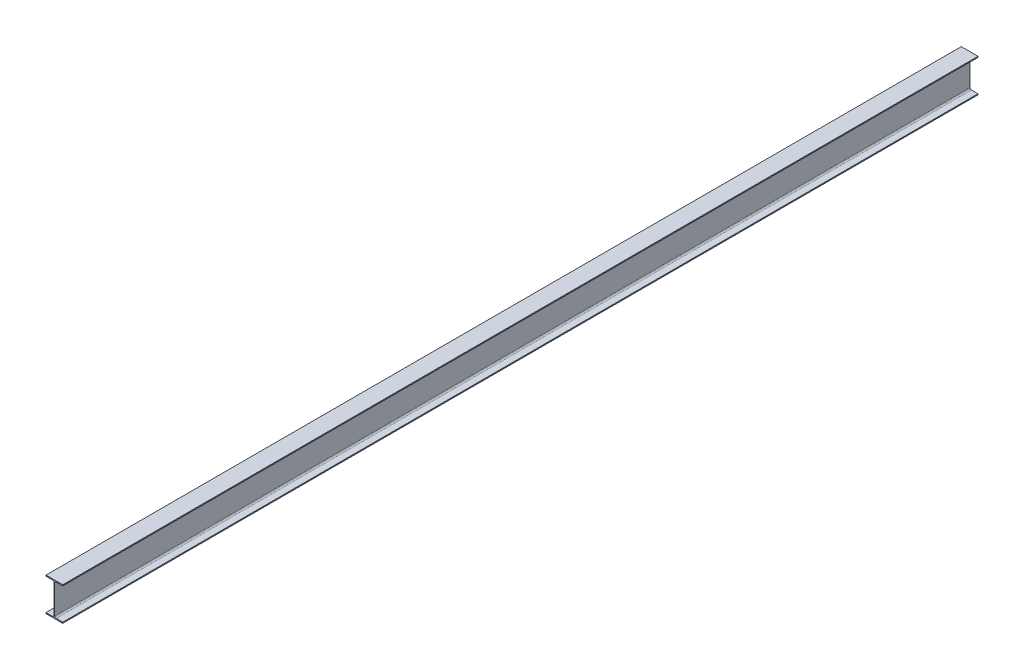
SolidWorks part; units mm, degrees
ref_plane "Front Plane" through (0, 0, 0) normal (0, 0, 1) x (1, 0, 0)
ref_plane "Top Plane" through (0, 0, 0) normal (0, 1, 0) x (1, 0, 0)
ref_plane "Right Plane" through (0, 0, 0) normal (1, 0, 0) x (0, 0, -1)
other "Configuration Table"
sketch "Sketch1" plane through (0, 0, 0) normal (0, 0, 1) x (1, 0, 0)
  line L0 (0, 0) -> (0, 300) construction
  line L1 (75, 0) -> (-75, 0)
  line L2 (-75, 0) -> (-75, 9)
  line L3 (-75, 9) -> (-16.25, 9)
  line L4 (3.25, 22) -> (3.25, 278)
  line L6 (-75, 291) -> (-75, 300)
  line L7 (-75, 300) -> (75, 300)
  line L8 (-3.25, 22) -> (-3.25, 278)
  line L9 (75, 291) -> (75, 300)
  line L10 (16.25, 291) -> (75, 291)
  line L11 (75, 9) -> (16.25, 9)
  line L12 (75, 0) -> (75, 9)
  line L13 (-16.25, 291) -> (-75, 291)
  arc A0 (16.25, 9) -> (3.25, 22) centre (16.25, 22) cw
  arc A1 (-3.25, 22) -> (-16.25, 9) centre (-16.25, 22) cw
  arc A2 (3.25, 278) -> (16.25, 291) centre (16.25, 278) cw
  arc A3 (-3.25, 278) -> (-16.25, 291) centre (-16.25, 278) ccw
  point P18 (3.25, 9)
  point P21 (-3.25, 9)
  point P24 (3.25, 291)
  point P27 (-3.25, 291)
  dimension "D6" = 13
  dimension "D1" = 300
  dimension "D2" = 150
  dimension "D3" = 6.5
  dimension "D4" = 9
  dimension "D5" = 9
extrude "Boss-Extrude1" add sketch "Sketch1" along normal blind 8210
